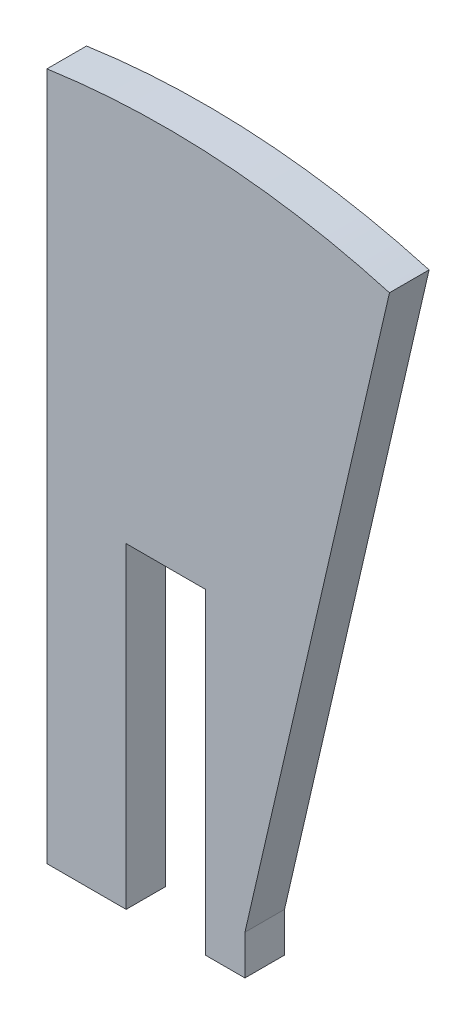
from build123d import *

# Parameters (mm, degrees)
BOSS_EXTRUDE1_DEPTH = 5
SKETCH2_W           = 20
SKETCH2_H           = 160
CUT_EXTRUDE1_DEPTH  = 10


with BuildPart() as part:
    # Sketch1 → Boss-Extrude1 (new, symmetric)
    with BuildSketch(Plane.XY):
        with BuildLine():
            Line((-30, 203.803827246), (-30, 30))
            Line((-30, 30), (20, 30))
            Line((20, 30), (20, 40))
            Line((20, 40), (56.500321431, 198.100261681))
            ThreePointArc((56.500321431, 198.100261681), (13.55357606, 205.553644035), (-30, 203.803827246))
        make_face()
    extrude(amount=BOSS_EXTRUDE1_DEPTH, both=True)

    # Sketch2 → Cut-Extrude1 (cut)
    with BuildSketch(Plane.XY.offset(5)):
        with Locations((0, 30)):
            Rectangle(SKETCH2_W, SKETCH2_H)
    extrude(amount=-CUT_EXTRUDE1_DEPTH, mode=Mode.SUBTRACT)


solid = part.part
